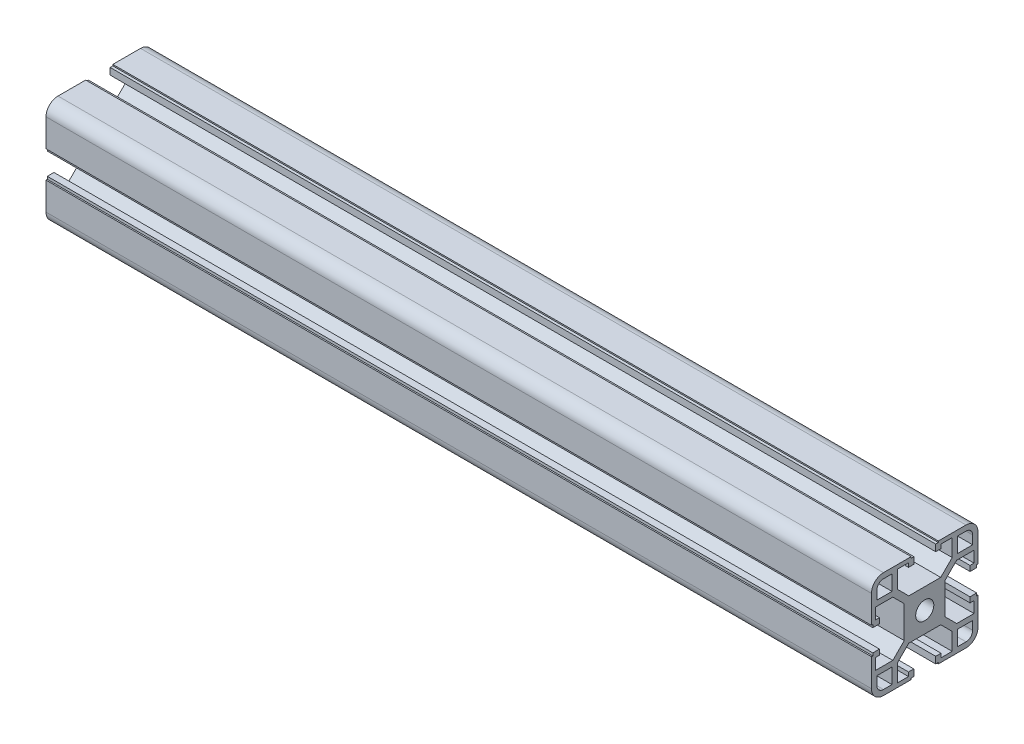
SolidWorks part; units mm, degrees
ref_plane "Front Plane" through (0, 0, 0) normal (0, 0, 1) x (1, 0, 0)
ref_plane "Top Plane" through (0, 0, 0) normal (0, 1, 0) x (1, 0, 0)
ref_plane "Right Plane" through (0, 0, 0) normal (1, 0, 0) x (0, 0, -1)
sketch "草图1" plane through (0, 0, 0) normal (0, 0, 1) x (1, 0, 0)
  line L0 (-984.975, 0) -> (-674.975, 0)
  dimension "D1" = 310
other "Aluminium profile 40 X 40B X R4.5(1)"
ref_plane "Plane1" through (-984.975, 0, 0) normal (1, 0, 0) x (0, 1, 0)
sketch "Sketch1" plane through (-984.975, 0, 0) normal (1, 0, 0) x (0, 1, 0)
  line L0 (-5.1, 20) -> (-5.1, 19.5)
  line L1 (-5.1, 19.5) -> (-4.1, 19.5)
  line L2 (-4.1, 19.5) -> (-4.1, 17)
  line L3 (-6.1, 18.5) -> (-10.3, 18.5)
  line L4 (-15.5, -20) -> (-5.1, -20)
  line L5 (-20, -15.5) -> (-20, -5.1)
  line L6 (15.5, 20) -> (5.1, 20)
  line L7 (20, 15.5) -> (20, 5.1)
  line L8 (0, 14.8756) -> (0, 0) construction
  line L9 (0, 0) -> (14.1675, 0) construction
  line L10 (-10.3, 18.5) -> (-10.3, 12)
  line L11 (-10.3, 12) -> (-6, 7.7)
  line L12 (-6, 7.7) -> (6, 7.7)
  line L13 (10.3, 12) -> (6, 7.7)
  line L14 (10.3, 18.5) -> (10.3, 12)
  line L15 (6.1, 18.5) -> (10.3, 18.5)
  line L16 (4.1, 19.5) -> (4.1, 17)
  line L17 (5.1, 19.5) -> (4.1, 19.5)
  line L18 (5.1, 20) -> (5.1, 19.5)
  line L19 (-5.1, 20) -> (-15.5, 20)
  line L20 (20, 5.1) -> (19.5, 5.1)
  line L21 (12.3, 18) -> (15.5, 18)
  line L22 (12.3, 18) -> (12.3, 12.3)
  line L23 (12.3, 12.3) -> (18, 12.3)
  line L24 (18, 15.5) -> (18, 12.3)
  line L25 (19.5, 5.1) -> (19.5, 4.1)
  line L26 (19.5, 4.1) -> (17, 4.1)
  line L27 (17, 6.1) -> (17, 4.1)
  line L28 (18.5, 6.1) -> (17, 6.1)
  line L29 (18.5, 6.1) -> (18.5, 10.3)
  line L30 (18.5, 10.3) -> (12, 10.3)
  line L31 (12, 10.3) -> (7.7, 6)
  line L32 (7.7, 6) -> (7.7, -6)
  line L33 (12, -10.3) -> (7.7, -6)
  line L34 (18.5, -10.3) -> (12, -10.3)
  line L35 (18.5, -6.1) -> (18.5, -10.3)
  line L36 (18.5, -6.1) -> (17, -6.1)
  line L37 (17, -4.1) -> (17, -6.1)
  line L38 (19.5, -4.1) -> (17, -4.1)
  line L39 (19.5, -5.1) -> (19.5, -4.1)
  line L40 (20, -5.1) -> (19.5, -5.1)
  line L41 (5.1, -20) -> (5.1, -19.5)
  line L42 (5.1, -19.5) -> (4.1, -19.5)
  line L43 (4.1, -19.5) -> (4.1, -17)
  line L44 (6.1, -17) -> (4.1, -17)
  line L45 (6.1, -18.5) -> (6.1, -17)
  line L46 (6.1, -18.5) -> (10.3, -18.5)
  line L47 (10.3, -18.5) -> (10.3, -12)
  line L48 (10.3, -12) -> (6, -7.7)
  line L49 (6, -7.7) -> (-6, -7.7)
  line L50 (-10.3, -12) -> (-6, -7.7)
  line L51 (-10.3, -18.5) -> (-10.3, -12)
  line L52 (-6.1, -18.5) -> (-10.3, -18.5)
  line L53 (-6.1, -18.5) -> (-6.1, -17)
  line L54 (-4.1, -17) -> (-6.1, -17)
  line L55 (-4.1, -19.5) -> (-4.1, -17)
  line L56 (-5.1, -19.5) -> (-4.1, -19.5)
  line L57 (-5.1, -20) -> (-5.1, -19.5)
  line L58 (-20, -5.1) -> (-19.5, -5.1)
  line L59 (5.1, -20) -> (15.5, -20)
  line L60 (-20, 5.1) -> (-20, 15.5)
  line L61 (-19.5, -5.1) -> (-19.5, -4.1)
  line L62 (-6.1, 18.5) -> (-6.1, 17)
  line L63 (-6.1, 17) -> (-4.1, 17)
  line L64 (6.1, 18.5) -> (6.1, 17)
  line L65 (4.1, 17) -> (6.1, 17)
  line L66 (-19.5, -4.1) -> (-17, -4.1)
  line L67 (-15.5, 18) -> (-12.3, 18)
  line L68 (-18, 15.5) -> (-18, 12.3)
  line L69 (-18, 12.3) -> (-12.3, 12.3)
  line L70 (-12.3, 18) -> (-12.3, 12.3)
  line L71 (-17, -6.1) -> (-17, -4.1)
  line L72 (-18.5, -6.1) -> (-17, -6.1)
  line L73 (-18.5, -6.1) -> (-18.5, -10.3)
  line L74 (-18.5, -10.3) -> (-12, -10.3)
  line L75 (-12, -10.3) -> (-7.7, -6)
  line L76 (-7.7, -6) -> (-7.7, 6)
  line L77 (-12, 10.3) -> (-7.7, 6)
  line L78 (-18.5, 10.3) -> (-12, 10.3)
  line L79 (-18.5, 6.1) -> (-18.5, 10.3)
  line L80 (-18.5, 6.1) -> (-17, 6.1)
  line L81 (-17, 4.1) -> (-17, 6.1)
  line L82 (-19.5, 4.1) -> (-17, 4.1)
  line L83 (-19.5, 5.1) -> (-19.5, 4.1)
  line L84 (-20, 5.1) -> (-19.5, 5.1)
  line L85 (20, -5.1) -> (20, -15.5)
  line L87 (-18, -12.3) -> (-12.3, -12.3)
  line L88 (-18, -12.3) -> (-18, -15.5)
  line L89 (-15.5, -18) -> (-12.3, -18)
  line L90 (-12.3, -12.3) -> (-12.3, -18)
  line L91 (12.3, -12.3) -> (18, -12.3)
  line L92 (12.3, -12.3) -> (12.3, -18)
  line L93 (12.3, -18) -> (15.5, -18)
  line L94 (18, -12.3) -> (18, -15.5)
  circle A0 centre (0, 0) radius 3.4
  arc A1 (-20, 15.5) -> (-15.5, 20) centre (-15.5, 15.5) cw
  arc A2 (20, 15.5) -> (15.5, 20) centre (15.5, 15.5) ccw
  arc A3 (-15.5, -20) -> (-20, -15.5) centre (-15.5, -15.5) cw
  arc A4 (15.5, -20) -> (20, -15.5) centre (15.5, -15.5) ccw
  arc A5 (-15.5, 18) -> (-18, 15.5) centre (-15.5, 15.5) ccw
  arc A6 (18, 15.5) -> (15.5, 18) centre (15.5, 15.5) ccw
  arc A7 (18, -15.5) -> (15.5, -18) centre (15.5, -15.5) cw
  arc A8 (-18, -15.5) -> (-15.5, -18) centre (-15.5, -15.5) ccw
  point P2 (0, 10)
  point P4 (0, 0)
  point P5 (-20, -20)
  point P6 (20, -20)
  point P7 (20, 20)
  point P8 (-20, 20)
  point P36 (-20, 20)
  point P39 (20, 20)
  point P121 (0, 0)
  dimension "D1" = 20.6
  dimension "D2" = 40
  dimension "D3" = 8.2
  dimension "D4" = 10.2
  dimension "D5" = 12.3
  dimension "D6" = 6.8
  dimension "D7" = 4.5
  dimension "D8" = 45
  dimension "D12" = 2
  dimension "D13" = 5.7
  dimension "D14" = 2
  dimension "D18" = 2.5
  dimension "D19" = 2.5
  dimension "D15" = 2.5
  dimension "D9" = 0.5
  dimension "D10" = 1.5
  dimension "D11" = 12
  dimension "D16" = 3
  dimension "D17" = 2
  dimension "D20" = 2
  dimension "D21" = 2
